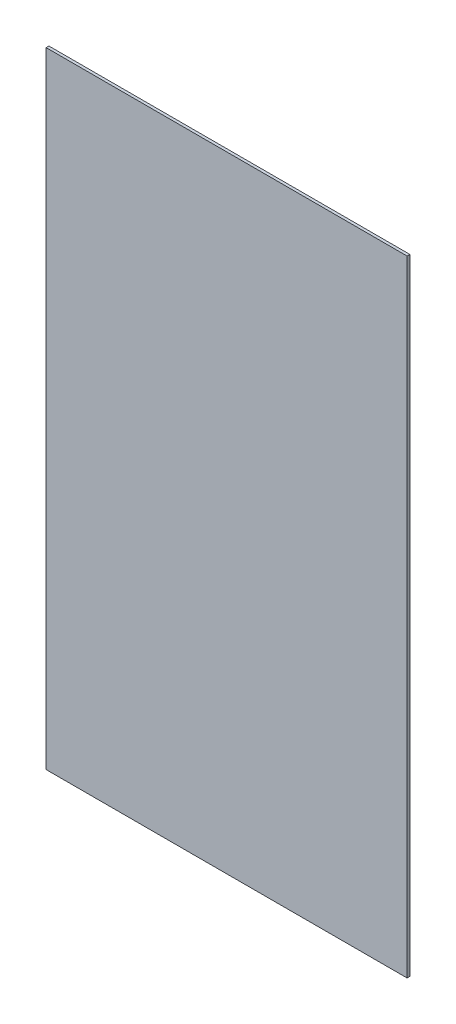
SolidWorks part; units mm, degrees
material "PMMA(有机玻璃)"
ref_plane "前视" through (0, 0, 0) normal (0, 0, 1) x (1, 0, 0)
ref_plane "上视" through (0, 0, 0) normal (0, 1, 0) x (1, 0, 0)
ref_plane "右视" through (0, 0, 0) normal (1, 0, 0) x (0, 0, -1)
sketch "草图1" plane through (0, 0, 0) normal (0, 0, 1) x (1, 0, 0)
  line L1 (-323, 559.5) -> (323, 559.5)
  line L2 (-323, 559.5) -> (-323, -559.5)
  line L3 (-323, -559.5) -> (323, -559.5)
  line L4 (323, 559.5) -> (323, -559.5)
  line L5 (-323, 559.5) -> (323, -559.5) construction
  line L6 (-323, -559.5) -> (323, 559.5) construction
  point P0 (0, 0)
  dimension "D1" = 1119
  dimension "D2" = 646
extrude "凸台-拉伸1" add sketch "草图1" along normal blind 5
